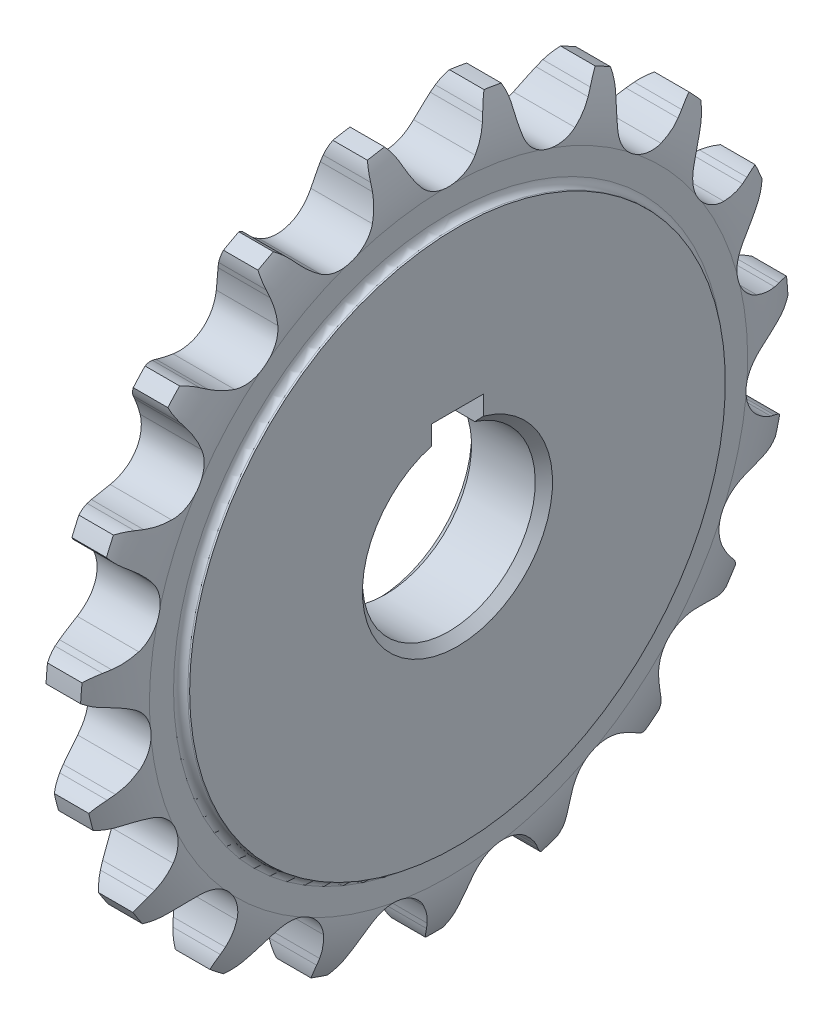
from build123d import *

# Parameters (mm, degrees)
CUT_EXTRUDE_1_DEPTH      = 4.685156443
PATTERN_CIRCULAR_1_COUNT = 19
SKETCH_4_W               = 6
SKETCH_4_H               = 3.260607938
CUT_EXTRUDE_2_DEPTH      = 59.686825317
CHAMFER_1_SIZE           = 1
CHAMFER_2_SIZE           = 1


with BuildPart() as part:
    # 草图1 → 旋转1 (revolve)
    with BuildSketch(Plane.XY, mode=Mode.PRIVATE) as revolve_1_sk:
        with BuildLine():
            Line((-4.685156443, 10), (-4.685156443, 31))
            Line((-4.685156443, 31), (-4.478175154, 31))
            ThreePointArc((-4.478175154, 31), (-3.892743663, 31.242493663), (-3.65025, 31.827925154))
            Line((-3.65025, 31.827925154), (-3.65025, 34.619639763))
            ThreePointArc((-3.65025, 34.619639763), (-3.245836945, 37.918781526), (-1.99925, 41))
            Line((-1.99925, 41), (1.99925, 41))
            ThreePointArc((1.99925, 41), (3.245836945, 37.918781526), (3.65025, 34.619639763))
            Line((3.65025, 34.619639763), (3.65025, 31.827925154))
            ThreePointArc((3.65025, 31.827925154), (3.892743663, 31.242493663), (4.478175154, 31))
            Line((4.478175154, 31), (4.685156443, 31))
            Line((4.685156443, 31), (4.685156443, 10))
            Line((4.685156443, 10), (-4.685156443, 10))
        make_face()
    revolve(revolve_1_sk.sketch.rotate(Axis((-6.35, 0, 0), (1, 0, 0)), 90), axis=Axis((-6.35, 0, 0), (1, 0, 0)))

    # 草图2 → 切除-拉伸1 (cut, symmetric)
    with BuildSketch(Plane(origin=(0, 0, 0), x_dir=(0, 0, -1), z_dir=(1, 0, 0))):
        with BuildLine():
            Line((4.552244709, 38.426451297), (4.858741585, 39.1448403))
            ThreePointArc((4.858741585, 39.1448403), (5.250930322, 39.90290393), (5.750855114, 40.594675334))
            ThreePointArc((5.750855114, 40.594675334), (0, 41), (-5.750855114, 40.594675334))
            ThreePointArc((-5.750855114, 40.594675334), (-5.250930322, 39.90290393), (-4.858741585, 39.1448403))
            Line((-4.858741585, 39.1448403), (-4.552244709, 38.426451297))
            ThreePointArc((-4.552244709, 38.426451297), (-3.937302758, 37.212676935), (-3.168676608, 36.089905522))
            ThreePointArc((-3.168676608, 36.089905522), (0, 34.549839763), (3.168676608, 36.089905522))
            ThreePointArc((3.168676608, 36.089905522), (3.937302758, 37.212676935), (4.552244709, 38.426451297))
        make_face()
    cut_extrude_1 = extrude(amount=CUT_EXTRUDE_1_DEPTH, both=True, mode=Mode.SUBTRACT)

    # 阵列(圆周)1: 切除-拉伸1 ×19 about axis
    pattern_circular_1_axis = Axis((0, 0, 0), (1, 0, 0))
    for i in range(1, PATTERN_CIRCULAR_1_COUNT):
        add(cut_extrude_1.rotate(pattern_circular_1_axis, i * 360 / PATTERN_CIRCULAR_1_COUNT), mode=Mode.SUBTRACT)

    # 草图4 → 切除-拉伸2 (cut, through all)
    with BuildSketch(Plane.ZY.offset(4.685156443)):
        with Locations((0, 11.169695983)):
            Rectangle(SKETCH_4_W, SKETCH_4_H)
    extrude(amount=-CUT_EXTRUDE_2_DEPTH, mode=Mode.SUBTRACT)

    # 倒角1
    chamfer_1_edges = [part.edges().sort_by_distance(p)[0] for p in [
        (-4.685156443, -10, 0),
    ]]
    chamfer(chamfer_1_edges, length=CHAMFER_1_SIZE)

    # 倒角2
    chamfer_2_edges = [part.edges().sort_by_distance(p)[0] for p in [
        (4.685156443, -10, 0),
    ]]
    chamfer(chamfer_2_edges, length=CHAMFER_2_SIZE)


solid = part.part
